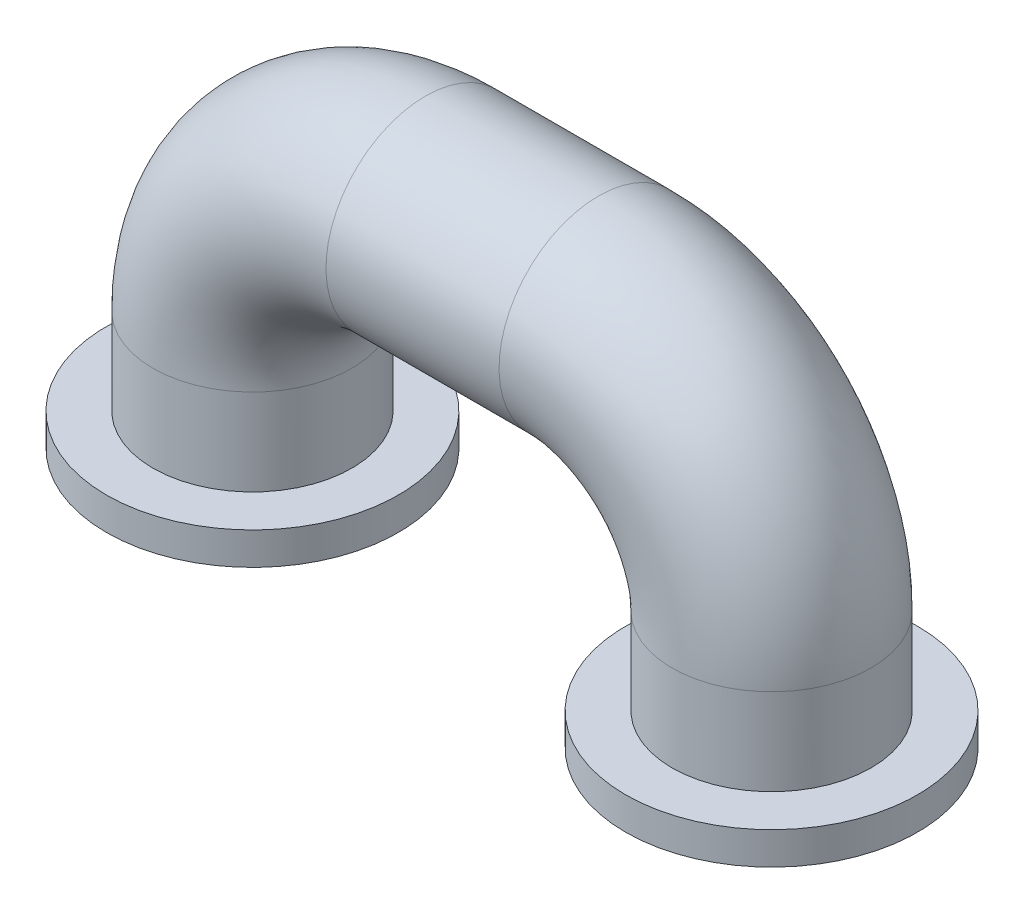
from build123d import *
from build123d.topology import SkipClean

# Parameters (mm, degrees)
SKETCH2_R           = 46
SKETCH2_R_2         = 40
SKETCH4_R           = 67.5
SKETCH4_R_2         = 40
BOSS_EXTRUDE1_DEPTH = 15


with BuildPart() as part:
    # Sweep1: sweep along a path in Sketch3
    with BuildLine(Plane.XY) as sweep1_path:
        Line((0, 0), (0, 40))
        ThreePointArc((0, 40), (23.431457505, 96.568542495), (80, 120))
        Line((80, 120), (160, 120))
        ThreePointArc((160, 120), (216.568542495, 96.568542495), (240, 40))
        Line((240, 40), (240, 0))
    # Sketch2 → Sweep1 (sweep)
    with BuildSketch(Plane(origin=(0, 0, 0), x_dir=(1, 0, 0), z_dir=(0, 1, 0))):
        Circle(SKETCH2_R)
        Circle(SKETCH2_R_2, mode=Mode.SUBTRACT)
    sweep(path=sweep1_path.line)

    # Sketch4 → Boss-Extrude1 (add)
    # profile 1 of 2: a face of its own
    with SkipClean():  # the faces are left unmerged after this step: merging them gives an invalid solid
        with BuildSketch(Plane(origin=(0, 0, 0), x_dir=(-1, 0, 0), z_dir=(0, -1, 0))):
            with Locations(Location((0, 0, 0), (0, 0, 90))):
                Circle(SKETCH4_R)
            Circle(SKETCH4_R_2, mode=Mode.SUBTRACT)
        # profile 2 of 2: a face of its own
        with BuildSketch(Plane(origin=(0, 0, 0), x_dir=(-1, 0, 0), z_dir=(0, -1, 0))):
            with Locations(Location((-240, 0, 0), (0, 0, 90))):
                Circle(SKETCH4_R)
            with Locations(Location((-240, 0, 0), (0, 0, 180))):
                Circle(SKETCH4_R_2, mode=Mode.SUBTRACT)
        extrude(amount=BOSS_EXTRUDE1_DEPTH)


solid = part.part
